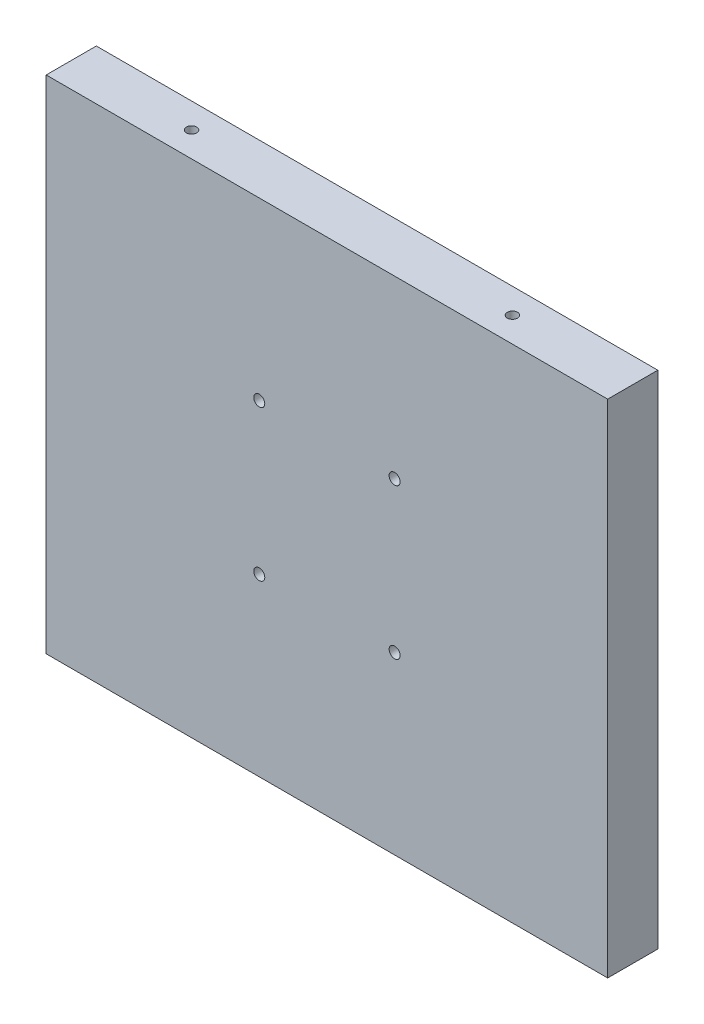
from build123d import *

# Parameters (mm, degrees)
SKETCH_1_W              = 560
SKETCH_1_H              = 500
EXTRUDE_1_DEPTH         = 50
HOLE_WIZARD_M12_1_D     = 10.2
HOLE_WIZARD_M12_1_DEPTH = 29.25
HOLE_WIZARD_M12_1_TIP   = 3.064389157
SKETCH_5_R              = 5.5
CUT_EXTRUDE_1_DEPTH     = 50


with BuildPart() as part:
    # 草图1 → 凸台-拉伸1 (new body)
    with BuildSketch(Plane.XY):
        Rectangle(SKETCH_1_W, SKETCH_1_H)
    extrude(amount=EXTRUDE_1_DEPTH)

    # M12 螺纹孔1
    with Locations(Plane(origin=(0, 250, 0), x_dir=(1, 0, 0), z_dir=(0, 1, 0))):
        with Locations((-160, -25), (160, -25)):
            Hole(HOLE_WIZARD_M12_1_D / 2, depth=HOLE_WIZARD_M12_1_DEPTH)
            with Locations((0, 0, -(HOLE_WIZARD_M12_1_DEPTH + HOLE_WIZARD_M12_1_TIP / 2))):  # 118° drill point
                Cone(0, HOLE_WIZARD_M12_1_D / 2, HOLE_WIZARD_M12_1_TIP, mode=Mode.SUBTRACT)

    # 草图5 → 切除-拉伸1 (cut)
    with BuildSketch(Plane.XY.offset(50)):
        with Locations((-67.5, 75)):
            Circle(SKETCH_5_R)
        with Locations((67.5, 75)):
            Circle(SKETCH_5_R)
        with Locations((67.5, -75)):
            Circle(SKETCH_5_R)
        with Locations((-67.5, -75)):
            Circle(SKETCH_5_R)
    extrude(amount=-CUT_EXTRUDE_1_DEPTH, mode=Mode.SUBTRACT)


solid = part.part
